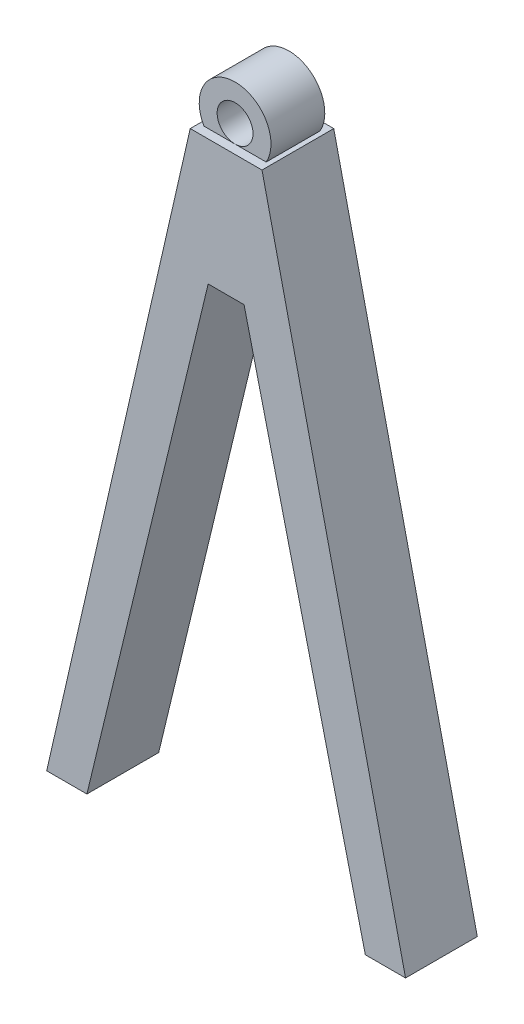
from build123d import *

# Parameters (mm, degrees)
BOSS_EXTRUDE1_DEPTH      = 150
BOSS_EXTRUDE1_DEPTH_BACK = 150
SKETCH1_R                = 200
SKETCH1_R_2              = 100
BOSS_EXTRUDE2_DEPTH      = 200
BOSS_EXTRUDE2_DEPTH_BACK = 200
CUT_EXTRUDE1_DEPTH       = 500
CUT_EXTRUDE1_DEPTH_BACK  = 500


with BuildPart() as part:
    # Sketch1 → Boss-Extrude1 (new, two sides: drawn at the far end of the back side and taken through both)
    with BuildSketch(Plane.XY.offset(-BOSS_EXTRUDE1_DEPTH_BACK)):
        Circle(SKETCH1_R)
        Circle(SKETCH1_R_2, mode=Mode.SUBTRACT)
    extrude(amount=BOSS_EXTRUDE1_DEPTH + BOSS_EXTRUDE1_DEPTH_BACK)

    # Sketch2 → Boss-Extrude2 (add, two sides: drawn at the far end of the back side and taken through both)
    with BuildSketch(Plane.XY.offset(-BOSS_EXTRUDE2_DEPTH_BACK)):
        Polygon((-200, -100), (200, -100), (1000, -3600), (-1000, -3600), align=None)
    extrude(amount=BOSS_EXTRUDE2_DEPTH + BOSS_EXTRUDE2_DEPTH_BACK)

    # Sketch3 → Cut-Extrude1 (cut, two sides: drawn at the far end of the back side and taken through both)
    with BuildSketch(Plane.XY.offset(200).offset(-CUT_EXTRUDE1_DEPTH_BACK)):
        Polygon((-100, -800), (100, -800), (800, -3700), (-800, -3700), align=None)
    extrude(amount=CUT_EXTRUDE1_DEPTH + CUT_EXTRUDE1_DEPTH_BACK, mode=Mode.SUBTRACT)


solid = part.part
